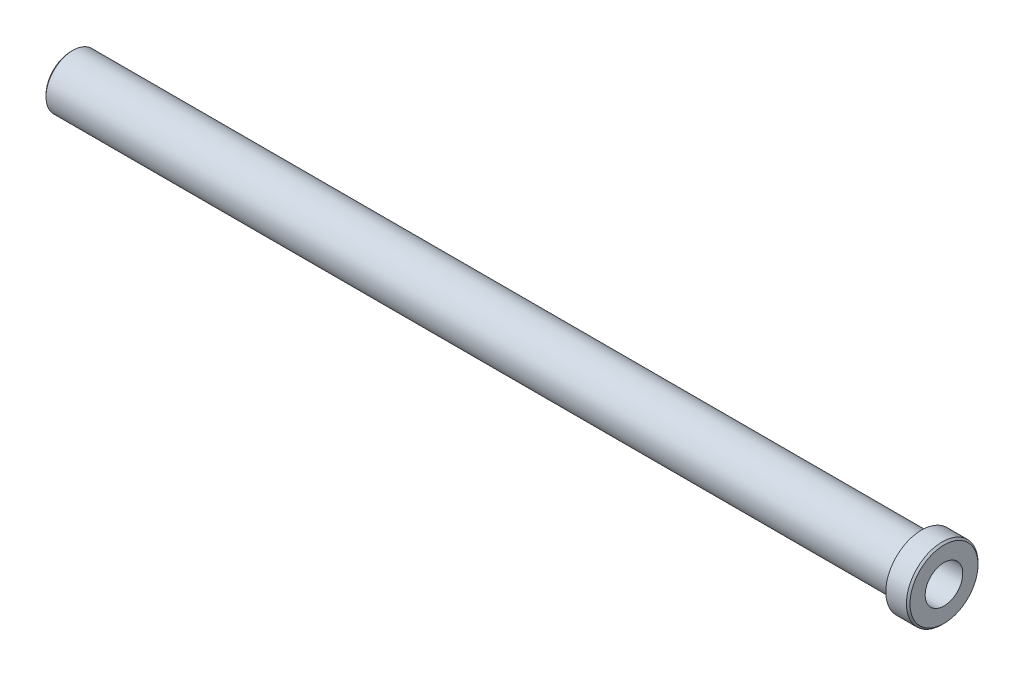
from build123d import *

# Parameters (mm, degrees)
SKETCH_1_R          = 30
EXTRUDE_1_DEPTH     = 475
SKETCH_2_R          = 40
EXTRUDE_2_DEPTH     = 25
CHAMFER_1_SIZE      = 2
FILLET_1_R          = 1
CUT_EXTRUDE_2_DEPTH = 120
SKETCH_5_R          = 21
CUT_EXTRUDE_3_DEPTH = 857.869301586
CHAMFER_2_SIZE      = 2
CHAMFER_3_SIZE      = 1


with BuildPart() as part:
    # 草图1 → 凸台-拉伸1 (new, symmetric)
    with BuildSketch(Plane(origin=(0, 0, 0), x_dir=(0, 0, -1), z_dir=(1, 0, 0))):
        with Locations(Location((0, 0, 0), (0, 0, 180))):
            Circle(SKETCH_1_R)
    extrude(amount=EXTRUDE_1_DEPTH, both=True)

    # 草图2 → 凸台-拉伸2 (add)
    with BuildSketch(Plane(origin=(475, 0, 0), x_dir=(0, 0, -1), z_dir=(1, 0, 0))):
        Circle(SKETCH_2_R)
    extrude(amount=EXTRUDE_2_DEPTH)

    # 倒角1
    chamfer_1_edges = [part.edges().sort_by_distance(p)[0] for p in [
        (500, 0, 40),
    ]]
    chamfer(chamfer_1_edges, length=CHAMFER_1_SIZE)

    # 圆角1
    fillet_1_edges = [part.edges().sort_by_distance(p)[0] for p in [
        (475, 0, -30),
    ]]
    fillet(fillet_1_edges, radius=FILLET_1_R)

    # 草图3 → 切除-拉伸2 (cut)
    with BuildSketch(Plane.ZY.offset(475)):
        with BuildLine():
            Line((0, -24.237375839), (0, 24.237375839))
            ThreePointArc((0, 24.237375839), (-2.61526925, 24.095865917), (-5.2, 23.672988564))
            Line((-5.2, 23.672988564), (-5.2, 20.346006979))
            ThreePointArc((-5.2, 20.346006979), (-8.03635208, 19.401470183), (-10.709844243, 18.063754767))
            Line((-10.709844243, 18.063754767), (-13.062375482, 20.416286007))
            ThreePointArc((-13.062375482, 20.416286007), (-17.138412814, 17.138412814), (-20.416286007, 13.062375482))
            Line((-20.416286007, 13.062375482), (-18.063754767, 10.709844243))
            ThreePointArc((-18.063754767, 10.709844243), (-19.401470183, 8.03635208), (-20.346006979, 5.2))
            Line((-20.346006979, 5.2), (-23.672988564, 5.2))
            ThreePointArc((-23.672988564, 5.2), (-24.237375839, 0), (-23.672988564, -5.2))
            Line((-23.672988564, -5.2), (-20.346006979, -5.2))
            ThreePointArc((-20.346006979, -5.2), (-19.401470183, -8.03635208), (-18.063754767, -10.709844243))
            Line((-18.063754767, -10.709844243), (-20.416286007, -13.062375482))
            ThreePointArc((-20.416286007, -13.062375482), (-17.138412814, -17.138412814), (-13.062375482, -20.416286007))
            Line((-13.062375482, -20.416286007), (-10.709844243, -18.063754767))
            ThreePointArc((-10.709844243, -18.063754767), (-8.03635208, -19.401470183), (-5.2, -20.346006979))
            Line((-5.2, -20.346006979), (-5.2, -23.672988564))
            ThreePointArc((-5.2, -23.672988564), (-2.61526925, -24.095865917), (0, -24.237375839))
        make_face()
        with BuildLine():
            ThreePointArc((5.2, 23.672988564), (2.61526925, 24.095865917), (0, 24.237375839))
            Line((0, 24.237375839), (0, -24.237375839))
            ThreePointArc((0, -24.237375839), (2.61526925, -24.095865917), (5.2, -23.672988564))
            Line((5.2, -23.672988564), (5.2, -20.346006979))
            ThreePointArc((5.2, -20.346006979), (8.03635208, -19.401470183), (10.709844243, -18.063754767))
            Line((10.709844243, -18.063754767), (13.062375482, -20.416286007))
            ThreePointArc((13.062375482, -20.416286007), (17.138412814, -17.138412814), (20.416286007, -13.062375482))
            Line((20.416286007, -13.062375482), (18.063754767, -10.709844243))
            ThreePointArc((18.063754767, -10.709844243), (19.401470183, -8.03635208), (20.346006979, -5.2))
            Line((20.346006979, -5.2), (23.672988564, -5.2))
            ThreePointArc((23.672988564, -5.2), (24.237375839, 0), (23.672988564, 5.2))
            Line((23.672988564, 5.2), (20.346006979, 5.2))
            ThreePointArc((20.346006979, 5.2), (19.401470183, 8.03635208), (18.063754767, 10.709844243))
            Line((18.063754767, 10.709844243), (20.416286007, 13.062375482))
            ThreePointArc((20.416286007, 13.062375482), (17.138412814, 17.138412814), (13.062375482, 20.416286007))
            Line((13.062375482, 20.416286007), (10.709844243, 18.063754767))
            ThreePointArc((10.709844243, 18.063754767), (8.03635208, 19.401470183), (5.2, 20.346006979))
            Line((5.2, 20.346006979), (5.2, 23.672988564))
        make_face()
    extrude(amount=-CUT_EXTRUDE_2_DEPTH, mode=Mode.SUBTRACT)

    # 草图5 → 切除-拉伸3 (cut, through all)
    with BuildSketch(Plane.ZY.offset(355)):
        Circle(SKETCH_5_R)
    extrude(amount=-CUT_EXTRUDE_3_DEPTH, mode=Mode.SUBTRACT)

    # 倒角2
    chamfer_2_edges = [part.edges().sort_by_distance(p)[0] for p in [
        (-475, 0, -30),
    ]]
    chamfer(chamfer_2_edges, length=CHAMFER_2_SIZE)

    # 倒角3
    chamfer_3_edges = [part.edges().sort_by_distance(p)[0] for p in [
        (-475, -24.237375839, 0),
        (-475, -19.401470183, 8.03635208),
        (-475, -17.138412814, 17.138412814),
        (-475, -8.03635208, 19.401470183),
        (-475, 0, 24.237375839),
        (-475, 8.03635208, 19.401470183),
        (-475, 17.138412814, 17.138412814),
        (-475, 19.401470183, 8.03635208),
        (-475, 24.237375839, 0),
        (-475, 19.401470183, -8.03635208),
        (-475, 17.138412814, -17.138412814),
        (-475, 8.03635208, -19.401470183),
        (-475, 0, -24.237375839),
        (-475, -8.03635208, -19.401470183),
        (-475, -17.138412814, -17.138412814),
        (-475, -19.401470183, -8.03635208),
    ]]
    chamfer(chamfer_3_edges, length=CHAMFER_3_SIZE)


solid = part.part
